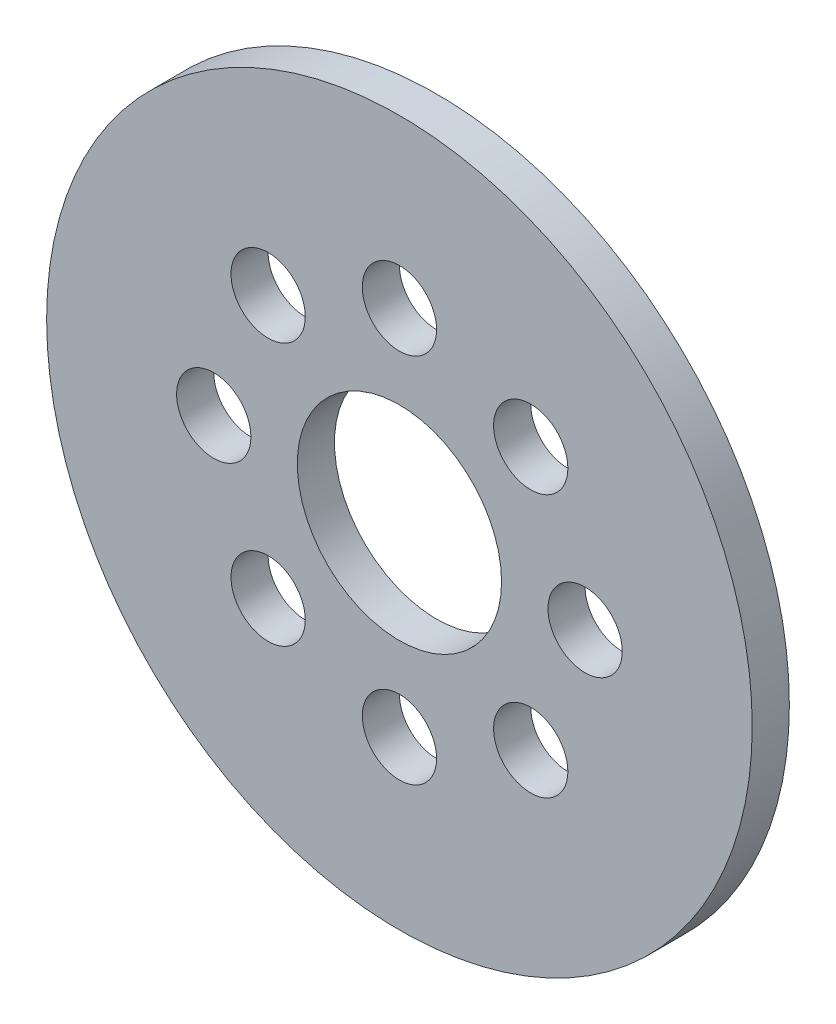
SolidWorks part; units mm, degrees
ref_plane "Front Plane" through (0, 0, 0) normal (0, 0, 1) x (1, 0, 0)
ref_plane "Top Plane" through (0, 0, 0) normal (0, 1, 0) x (1, 0, 0)
ref_plane "Right Plane" through (0, 0, 0) normal (1, 0, 0) x (0, 0, -1)
other "Configuration Table"
sketch "Sketch2" plane through (0, 0, 0) normal (0, 0, 1) x (1, 0, 0)
  circle A0 centre (0, 0) radius 95
  circle A1 centre (0, 0) radius 27.5
  dimension "D1" = 190
  dimension "D2" = 55
extrude "Boss-Extrude1" add sketch "Sketch2" along normal blind 10
sketch "Sketch3" plane through (0, 0, 10) normal (0, 0, 1) x (1, 0, 0)
  circle A0 centre (50, 0) radius 10
extrude "Cut-Extrude1" cut sketch "Sketch3" against normal through all both and the other way through all
pattern_circular "CirPattern1" count 8 over 360 about axis through (0, 0, 0) along (0, 0, 1) of "Cut-Extrude1"
